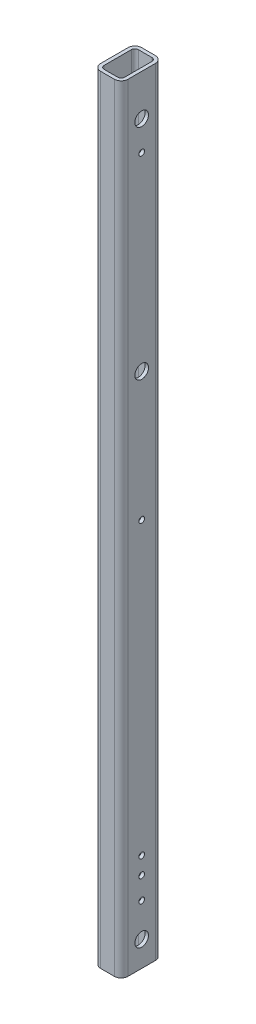
from build123d import *

# Parameters (mm, degrees)
F_30X20X2_5_1_DEPTH = 568
CUT_EXTRUDE_1_REACH = 570.55
SKETCH_6_R          = 10.5
HOLE_WIZARD_M8_1_D  = 10
HOLE_WIZARD_M5_1_D  = 4.2


with BuildPart() as part:
    # Sketch14 → 矩型管 30X20X2.5(1) (new body)
    with BuildSketch(Plane(origin=(0, 0, 0), x_dir=(-1, 0, 0), z_dir=(0, 1, 0))):
        with BuildLine():
            Line((-5, -15), (5, -15))
            ThreePointArc((5, -15), (8.535533906, -13.535533906), (10, -10))
            Line((10, -10), (10, 10))
            ThreePointArc((10, 10), (8.535533906, 13.535533906), (5, 15))
            Line((5, 15), (-5, 15))
            ThreePointArc((-5, 15), (-8.535533906, 13.535533906), (-10, 10))
            Line((-10, 10), (-10, -10))
            ThreePointArc((-10, -10), (-8.535533906, -13.535533906), (-5, -15))
        make_face()
        with BuildLine():
            Line((-5, -12.5), (5, -12.5))
            ThreePointArc((5, -12.5), (6.767766953, -11.767766953), (7.5, -10))
            Line((7.5, -10), (7.5, 10))
            ThreePointArc((7.5, 10), (6.767766953, 11.767766953), (5, 12.5))
            Line((5, 12.5), (-5, 12.5))
            ThreePointArc((-5, 12.5), (-6.767766953, 11.767766953), (-7.5, 10))
            Line((-7.5, 10), (-7.5, -10))
            ThreePointArc((-7.5, -10), (-6.767766953, -11.767766953), (-5, -12.5))
        make_face(mode=Mode.SUBTRACT)
    extrude(amount=F_30X20X2_5_1_DEPTH)

    # 草图6 → 切除-拉伸1 (cut, up to next)
    with BuildSketch(Plane.ZY.offset(10), mode=Mode.PRIVATE) as cut_extrude_1_sk1:
        with Locations(Location((0, 18.5, 0), (0, 0, 17.752790162))):
            Circle(SKETCH_6_R)
    cut_extrude_1_tool1 = extrude(cut_extrude_1_sk1.sketch, amount=-CUT_EXTRUDE_1_REACH, mode=Mode.PRIVATE) & part.part
    add(cut_extrude_1_tool1.solids().sort_by_distance((-10, 18.5, 0))[0], mode=Mode.SUBTRACT)

    # M8 间隙孔1 (through all)
    with Locations(Plane.ZY.offset(10)):
        with Locations((0, 538), (0, 378), (0, 18.5)):
            Hole(HOLE_WIZARD_M8_1_D / 2)

    # M5 螺纹孔1 (through all)
    with Locations(Plane(origin=(10, 0, 0), x_dir=(0, 0, -1), z_dir=(1, 0, 0))):
        with Locations((0, 516.5), (0, 284), (0, 71.5), (0, 59), (0, 43)):
            Hole(HOLE_WIZARD_M5_1_D / 2)


solid = part.part
